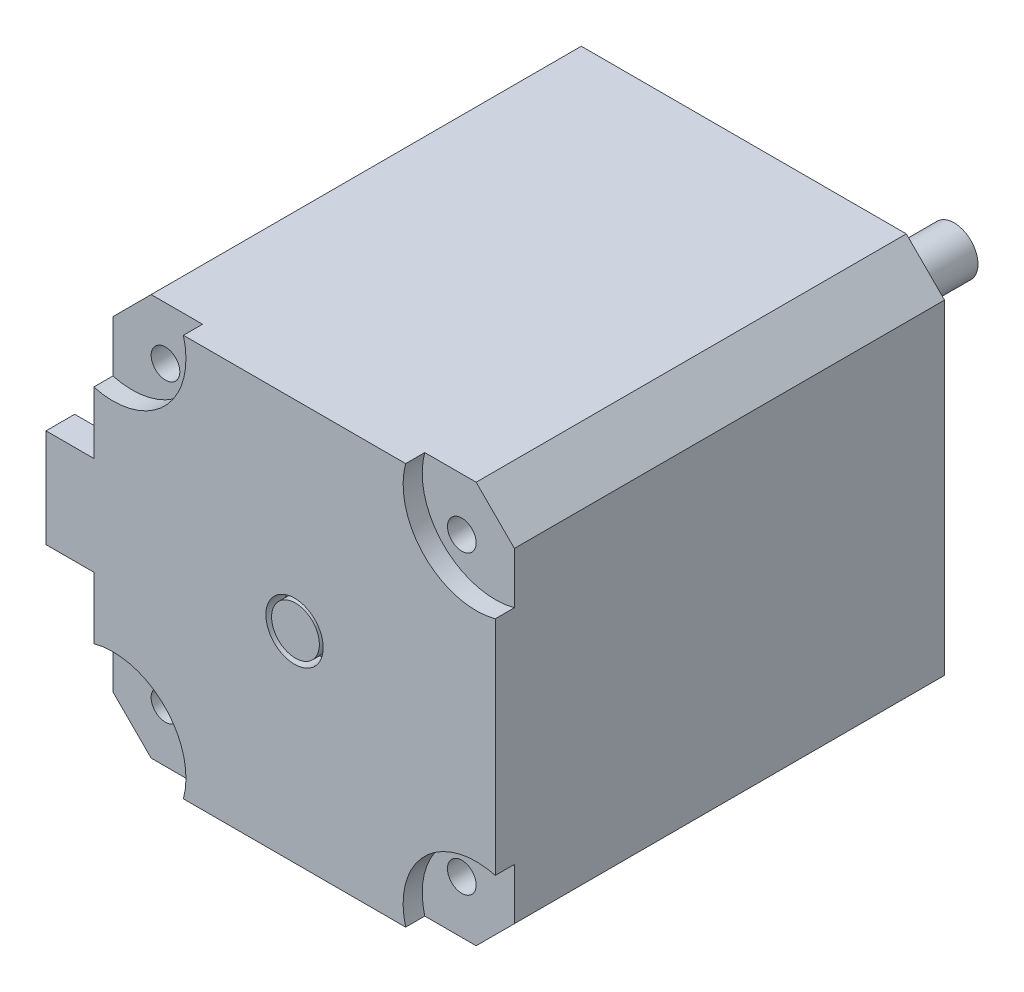
from build123d import *

# Parameters (mm, degrees)
SKETCH1_W           = 42
SKETCH1_H           = 42
SKETCH1_R           = 1.5
BOSS_EXTRUDE1_DEPTH = 47
CUT_EXTRUDE1_DEPTH  = 56.596762496
SKETCH4_R           = 11
BOSS_EXTRUDE2_DEPTH = 2
BOSS_EXTRUDE3_DEPTH = 20
CUT_EXTRUDE2_DEPTH  = 2
SKETCH8_R           = 3
CUT_EXTRUDE3_DEPTH  = 2
BOSS_EXTRUDE4_START = 1.9
SKETCH9_R           = 2.5
BOSS_EXTRUDE4_DEPTH = 1.9
SKETCH10_W          = 3
SKETCH10_H          = 10.31009041
SKETCH10_W_2        = 2.478607588
SKETCH10_H_2        = 8.518222776
BOSS_EXTRUDE5_DEPTH = 5
SKETCH11_R          = 0.5
BOSS_EXTRUDE6_DEPTH = 5


with BuildPart() as part:
    # Sketch1 → Boss-Extrude1 (new body)
    with BuildSketch(Plane.XY):
        Rectangle(SKETCH1_W, SKETCH1_H)
        with Locations((-15.5, 15.5)):
            Circle(SKETCH1_R, mode=Mode.SUBTRACT)
        with Locations(Location((15.5, 15.5, 0), (0, 0, 180))):
            Circle(SKETCH1_R, mode=Mode.SUBTRACT)
        with Locations(Location((-15.5, -15.5, 0), (0, 0, 180))):
            Circle(SKETCH1_R, mode=Mode.SUBTRACT)
        with Locations((15.5, -15.5)):
            Circle(SKETCH1_R, mode=Mode.SUBTRACT)
    extrude(amount=BOSS_EXTRUDE1_DEPTH)

    # Sketch3 → Cut-Extrude1 (cut, through all)
    with BuildSketch(Plane(origin=(0, 0, 0), x_dir=(-1, 0, 0), z_dir=(0, 0, -1))):
        Polygon((-21, 17), (-17, 21), (-21, 21), align=None)
        Polygon((21, 21), (17, 21), (21, 17), align=None)
        Polygon((21, -17), (17, -21), (21, -21), align=None)
        Polygon((-21, -21), (-17, -21), (-21, -17), align=None)
    extrude(amount=-CUT_EXTRUDE1_DEPTH, mode=Mode.SUBTRACT)

    # Sketch4 → Boss-Extrude2 (add)
    with BuildSketch(Plane(origin=(0, 0, 0), x_dir=(-1, 0, 0), z_dir=(0, 0, -1))):
        Circle(SKETCH4_R)
    extrude(amount=BOSS_EXTRUDE2_DEPTH)

    # Sketch5 → Boss-Extrude3 (add)
    with BuildSketch(Plane(origin=(0, 0, -2), x_dir=(-1, 0, 0), z_dir=(0, 0, -1))):
        with BuildLine():
            Line((1.7, -1.833030278), (1.7, 1.833030278))
            ThreePointArc((1.7, 1.833030278), (-2.5, 0), (1.7, -1.833030278))
        make_face()
    extrude(amount=BOSS_EXTRUDE3_DEPTH)

    # Sketch7 → Cut-Extrude2 (cut)
    with BuildSketch(Plane.XY.offset(47)):
        with BuildLine():
            Line((21, 17), (21, 11.625484678))
            ThreePointArc((21, 11.625484678), (13.597062084, 13.597062084), (11.625484678, 21))
            Line((11.625484678, 21), (17, 21))
            Line((17, 21), (21, 17))
        make_face()
        with BuildLine():
            Line((-21, -17), (-21, -11.625484678))
            ThreePointArc((-21, -11.625484678), (-13.597062084, -13.597062084), (-11.625484678, -21))
            Line((-11.625484678, -21), (-17, -21))
            Line((-17, -21), (-21, -17))
        make_face()
        with BuildLine():
            Line((-11.625484678, 21), (-17, 21))
            Line((-17, 21), (-21, 17))
            Line((-21, 17), (-21, 11.625484678))
            ThreePointArc((-21, 11.625484678), (-13.597062084, 13.597062084), (-11.625484678, 21))
        make_face()
        with BuildLine():
            Line((11.625484678, -21), (17, -21))
            Line((17, -21), (21, -17))
            Line((21, -17), (21, -11.625484678))
            ThreePointArc((21, -11.625484678), (13.597062084, -13.597062084), (11.625484678, -21))
        make_face()
    extrude(amount=-CUT_EXTRUDE2_DEPTH, mode=Mode.SUBTRACT)

    # Sketch8 → Cut-Extrude3 (cut)
    with BuildSketch(Plane.XY.offset(47)):
        Circle(SKETCH8_R)
    extrude(amount=-CUT_EXTRUDE3_DEPTH, mode=Mode.SUBTRACT)

    # Sketch9 → Boss-Extrude4 (add)
    with BuildSketch(Plane.XY.offset(45).offset(BOSS_EXTRUDE4_START)):
        with Locations(Location((0, 0, 0), (0, 0, 180))):
            Circle(SKETCH9_R)
    extrude(amount=-BOSS_EXTRUDE4_DEPTH)

    # Sketch10 → Boss-Extrude5 (add)
    with BuildSketch(Plane.ZY.offset(21)):
        with Locations((45.5, 0)):
            Rectangle(SKETCH10_W, SKETCH10_H)
        with Locations((45.5, 0)):
            Rectangle(SKETCH10_W_2, SKETCH10_H_2, mode=Mode.SUBTRACT)
    extrude(amount=BOSS_EXTRUDE5_DEPTH)

    # Sketch11 → Boss-Extrude6 (add)
    with BuildSketch(Plane.ZY.offset(21)):
        with Locations(Location((45.5, 3.127782029, 0), (0, 0, 180))):
            Circle(SKETCH11_R)
        with Locations(Location((45.5, 1.627782029, 0), (0, 0, 180))):
            Circle(SKETCH11_R)
        with Locations(Location((45.5, 0.127782029, 0), (0, 0, 180))):
            Circle(SKETCH11_R)
        with Locations(Location((45.5, -1.372217971, 0), (0, 0, 180))):
            Circle(SKETCH11_R)
        with Locations(Location((45.5, -2.872217971, 0), (0, 0, 180))):
            Circle(SKETCH11_R)
    extrude(amount=BOSS_EXTRUDE6_DEPTH)


solid = part.part
